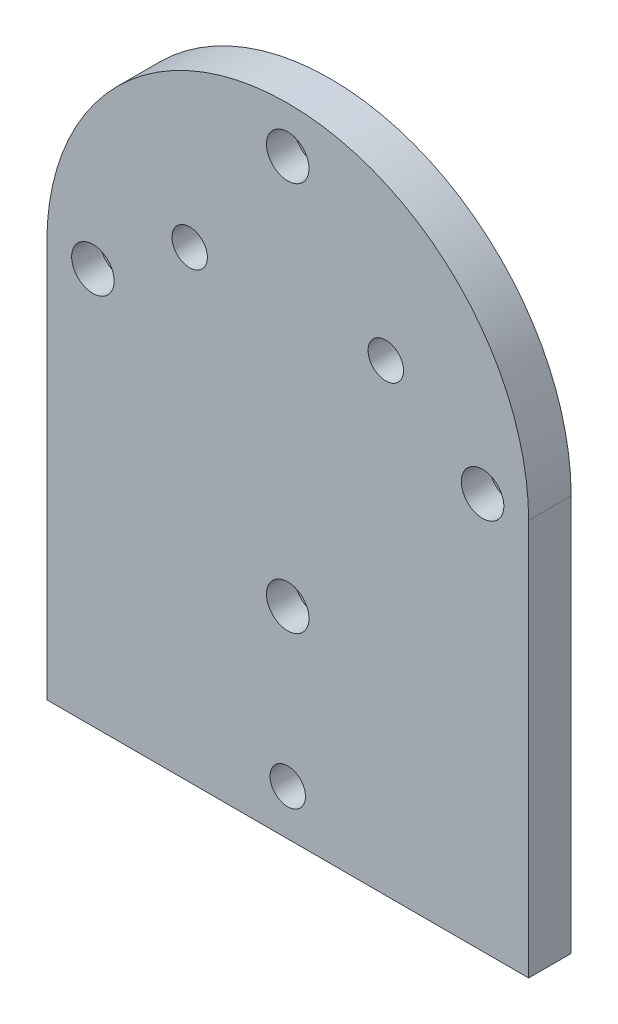
SolidWorks part; units mm, degrees
ref_plane "Front Plane" through (0, 0, 0) normal (0, 0, 1) x (1, 0, 0)
ref_plane "Top Plane" through (0, 0, 0) normal (0, 1, 0) x (1, 0, 0)
ref_plane "Right Plane" through (0, 0, 0) normal (1, 0, 0) x (0, 0, -1)
other "Configuration Table"
sketch "Sketch2" plane through (0, 0, 0) normal (0, 0, 1) x (1, 0, 0)
  line L0 (2.1816, 9.7439) -> (2.1816, -46.1827)
  line L1 (2.1816, -46.1827) -> (-65.8184, -46.1827)
  line L2 (-65.8184, -46.1827) -> (-65.8184, 9.7439)
  arc A0 (2.1816, 9.7439) -> (-65.8184, 9.7439) centre (-31.8184, 9.7439) ccw
  dimension "D1" = 68
extrude "Boss-Extrude1" add sketch "Sketch2" along normal blind 6
sketch "Sketch3" plane through (0, 0, 6) normal (0, 0, 1) x (1, 0, 0)
  circle A0 centre (-31.8184, 9.7439) radius 27.5
  circle A1 centre (-4.3184, 9.7439) radius 3
  circle A2 centre (-31.8184, -17.7561) radius 3
  circle A3 centre (-59.3184, 9.7439) radius 3
  circle A4 centre (-31.8184, 37.2439) radius 3
  point P14 (-31.8184, 9.7439)
  dimension "D1" = 55
  dimension "D2" = 6
  dimension "D3" = 4
extrude "Cut-Extrude1" cut sketch "Sketch3" against normal blind 4 contours A0 A4 | A0 A4 | A0 A1 | A0 A1 | A0 A3 | A0 A2 | A0 A2
sketch "Sketch6" plane through (0, 0, 6) normal (0, 0, 1) x (1, 0, 0)
  circle A0 centre (-30.714, 3.4856) radius 7.3426
sketch "Sketch9" plane through (0, 0, 0) normal (0, 0, -1) x (-1, 0, 0)
  circle A0 centre (45.6585, 19.2102) radius 2.5
  circle A1 centre (17.9783, 19.2102) radius 2.5
  circle A2 centre (31.8184, -39.7538) radius 2.5
extrude "Cut-Extrude2" cut sketch "Sketch9" against normal blind 6
